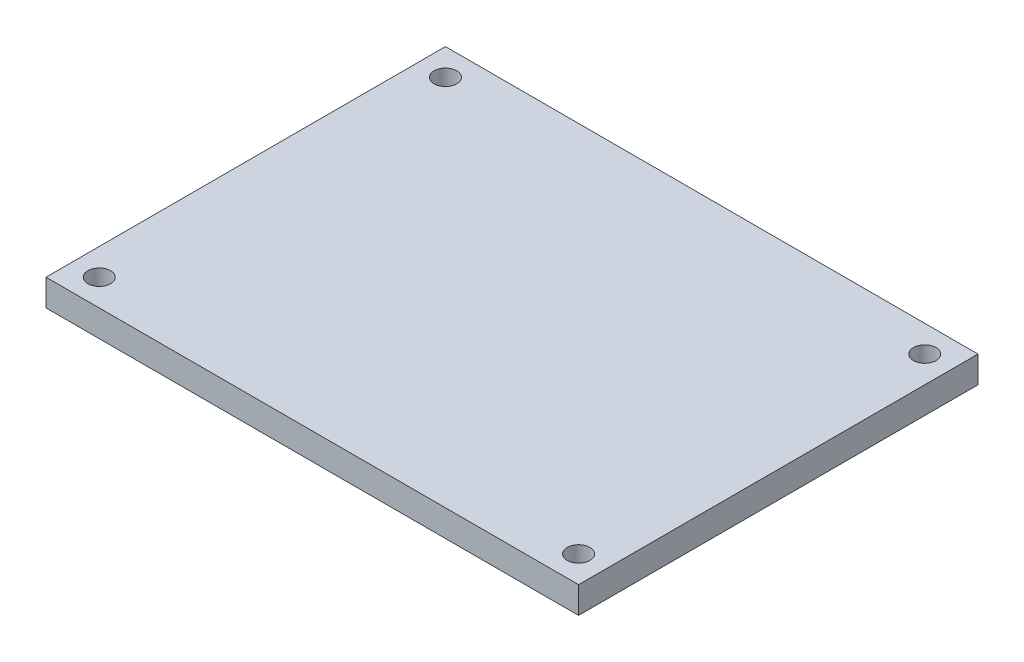
from build123d import *

# Parameters (mm, degrees)
SKETCH_1_W          = 200
SKETCH_1_H          = 150
EXTRUDE_1_DEPTH     = 10
HOLE_WIZARD_M10_1_D = 8.5


with BuildPart() as part:
    # 草图1 → 凸台-拉伸1 (new body)
    with BuildSketch(Plane(origin=(0, 0, 0), x_dir=(1, 0, 0), z_dir=(0, 1, 0))):
        Rectangle(SKETCH_1_W, SKETCH_1_H)
    extrude(amount=EXTRUDE_1_DEPTH)

    # M10 螺纹孔1 (through all)
    with Locations(Plane(origin=(0, 0, 0), x_dir=(-1, 0, 0), z_dir=(0, -1, 0))):
        with Locations((90, -65), (90, 65), (-90, 65), (-90, -65)):
            Hole(HOLE_WIZARD_M10_1_D / 2)


solid = part.part
